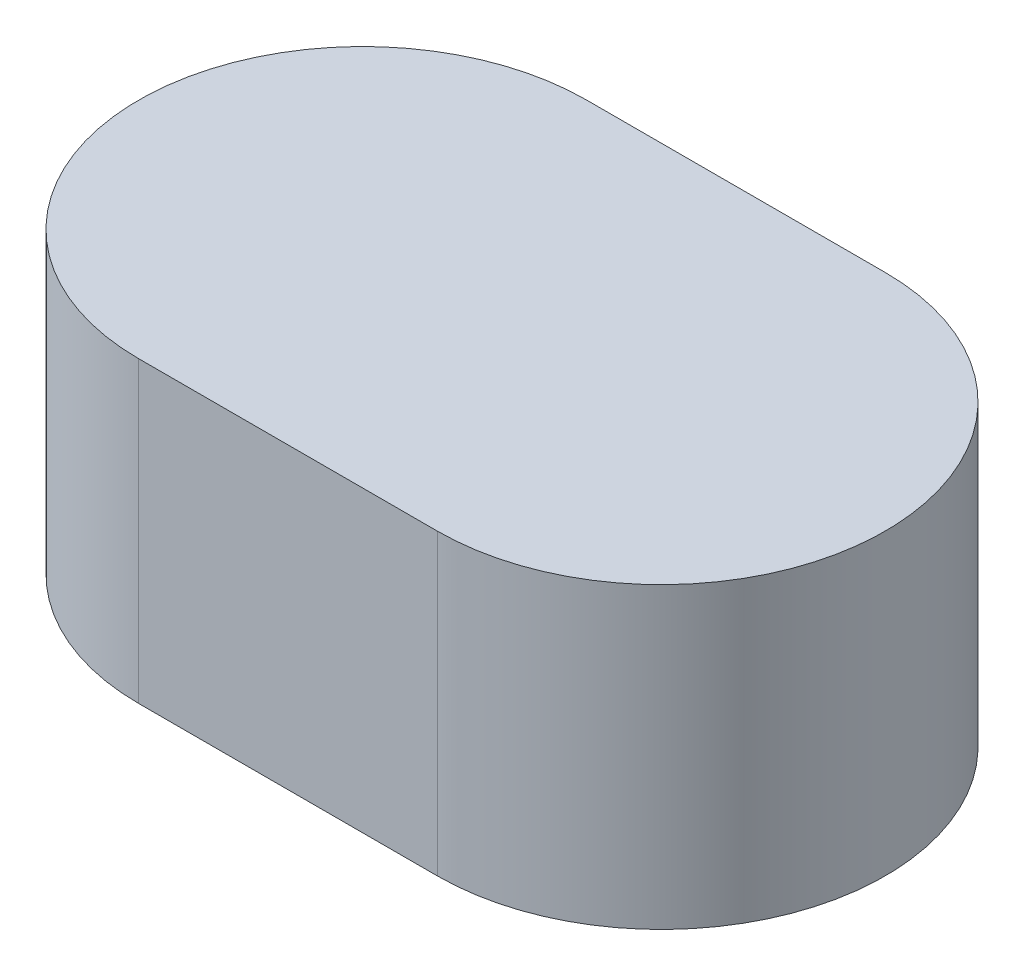
from build123d import *

# Parameters (mm, degrees)
BOSS_EXTRUDE1_DEPTH = 8


with BuildPart() as part:
    # Sketch1 → Boss-Extrude1 (new body)
    with BuildSketch(Plane(origin=(0, 0, 0), x_dir=(1, 0, 0), z_dir=(0, 1, 0))):
        with BuildLine():
            Line((-4, 6), (4, 6))
            ThreePointArc((4, 6), (10, 0), (4, -6))
            Line((4, -6), (-4, -6))
            ThreePointArc((-4, -6), (-10, 0), (-4, 6))
        make_face()
    extrude(amount=BOSS_EXTRUDE1_DEPTH)


solid = part.part
